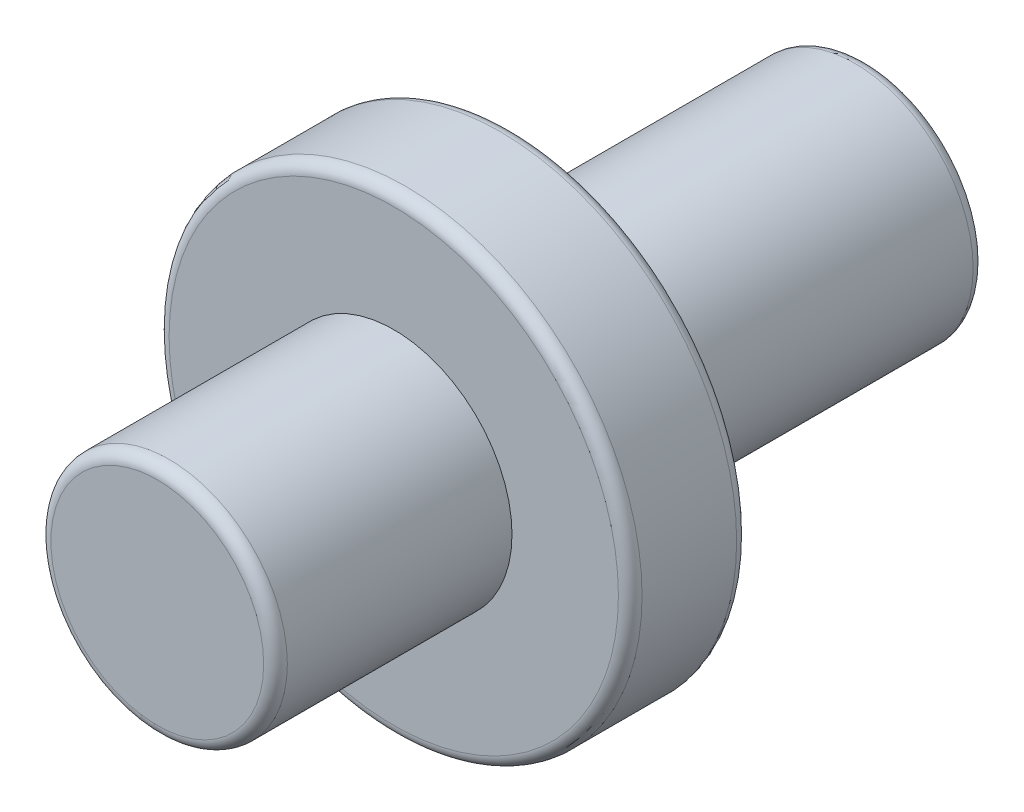
from build123d import *

# Parameters (mm, degrees)
SKETCH_1_R      = 2
EXTRUDE_1_DEPTH = 6
SKETCH_2_R      = 4
EXTRUDE_2_DEPTH = 2
SKETCH_3_R      = 2
EXTRUDE_3_DEPTH = 4
FILLET_1_R      = 0.2
FILLET_2_R      = 0.2


with BuildPart() as part:
    # 草图1 → 凸台-拉伸1 (new body)
    with BuildSketch(Plane.XY):
        Circle(SKETCH_1_R)
    extrude(amount=EXTRUDE_1_DEPTH)

    # 草图2 → 凸台-拉伸2 (add)
    with BuildSketch(Plane.XY.offset(6)):
        Circle(SKETCH_2_R)
    extrude(amount=EXTRUDE_2_DEPTH)

    # 草图3 → 凸台-拉伸3 (add)
    with BuildSketch(Plane.XY.offset(8)):
        Circle(SKETCH_3_R)
    extrude(amount=EXTRUDE_3_DEPTH)

    # 圆角1
    fillet_1_edges = [part.edges().sort_by_distance(p)[0] for p in [
        (-2, 0, 12),
        (-2, 0, 0),
    ]]
    fillet(fillet_1_edges, radius=FILLET_1_R)

    # 圆角2
    fillet_2_edges = [part.edges().sort_by_distance(p)[0] for p in [
        (-4, 0, 6),
        (-4, 0, 8),
    ]]
    fillet(fillet_2_edges, radius=FILLET_2_R)


solid = part.part
